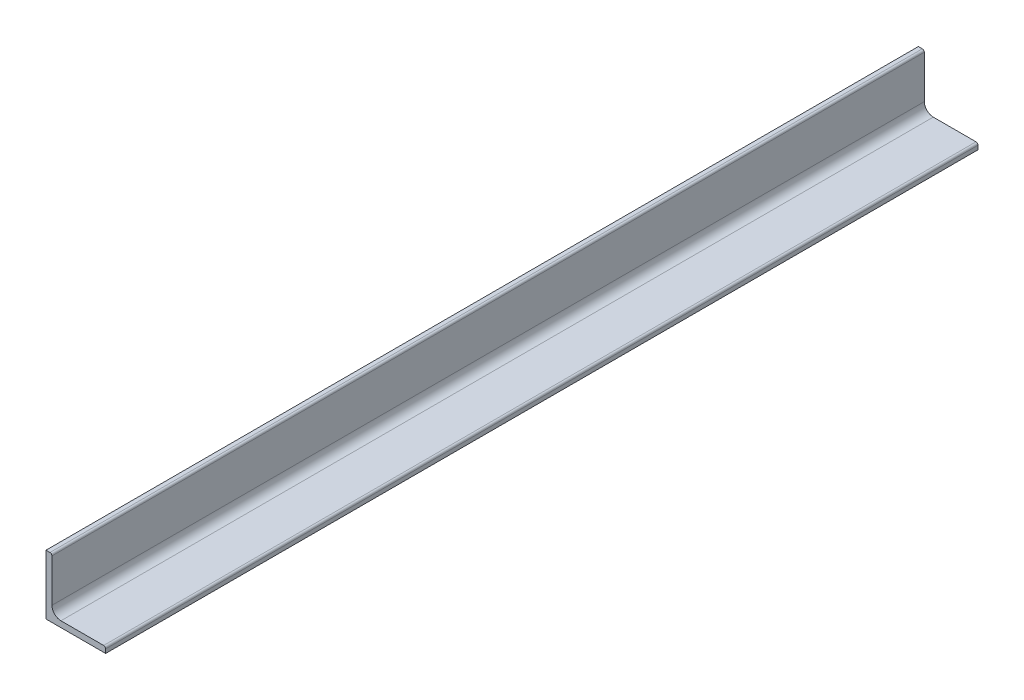
SolidWorks part; units mm, degrees
material "Plain Carbon Steel"
ref_plane "Plane1" through (0, 0, 0) normal (0, 0, 1) x (1, 0, 0)
ref_plane "Plane2" through (0, 0, 0) normal (0, 1, 0) x (1, 0, 0)
ref_plane "Plane3" through (0, 0, 0) normal (1, 0, 0) x (0, 0, -1)
sketch "Sketch1" plane through (0, 0, 0) normal (0, 0, 1) x (1, 0, 0)
  line L0 (0, 0) -> (0, 30)
  line L1 (0, 15) -> (3, 15) construction
  line L2 (3, 29) -> (3, 7.5)
  line L3 (7.5, 3) -> (29, 3)
  line L4 (15, 3) -> (15, 0) construction
  line L5 (30, 0) -> (0, 0)
  line L6 (0, 30) -> (2, 30)
  line L7 (30, 0) -> (30, 2)
  arc A0 (30, 2) -> (29, 3) centre (29, 2) ccw
  arc A1 (2, 30) -> (3, 29) centre (2, 29) cw
  arc A2 (7.5, 3) -> (3, 7.5) centre (7.5, 7.5) cw
  point P10 (15, 0)
  point P14 (0, 15)
  point P15 (3, 15)
  point P16 (15, 3)
  point P17 (3, 30)
  point P18 (30, 3)
  point P21 (30, 3)
  point P24 (3, 30)
extrude "Boss-Extrude1" add sketch "Sketch1" along normal mid plane 438.8 contours L2 A2 L3 A0 L7 L5 L0 L6 A1
equation "\"D2@Sketch1\" = \"D1@Sketch1\" / 3"
